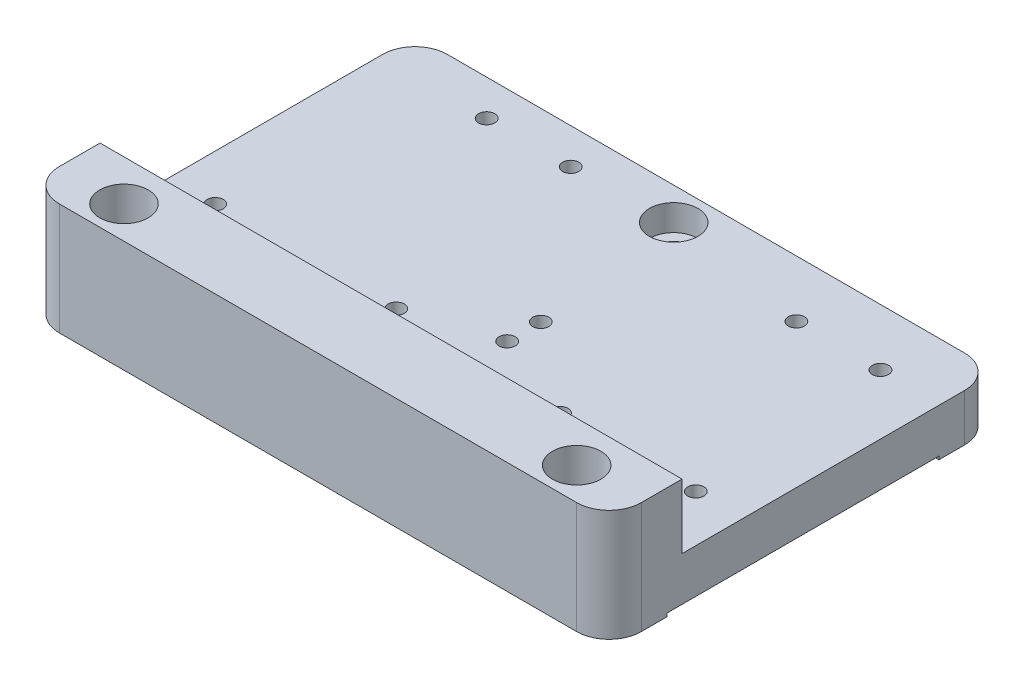
SolidWorks part; units mm, degrees
ref_plane "Front Plane" through (0, 0, 0) normal (0, 0, 1) x (1, 0, 0)
ref_plane "Top Plane" through (0, 0, 0) normal (0, 1, 0) x (1, 0, 0)
ref_plane "Right Plane" through (0, 0, 0) normal (1, 0, 0) x (0, 0, -1)
sketch "Sketch1" plane through (0, 0, 0) normal (0, 1, 0) x (1, 0, 0)
  line L1 (-73.3594, 57.0703) -> (16.6406, 57.0703)
  line L2 (-73.3594, 57.0703) -> (-73.3594, -2.9297)
  line L3 (-73.3594, -2.9297) -> (16.6406, -2.9297)
  line L4 (16.6406, 57.0703) -> (16.6406, -2.9297)
  dimension "D1" = 90
  dimension "D2" = 60
extrude "Boss-Extrude1" add sketch "Sketch1" along normal blind 7.3
sketch "Sketch2" plane through (0, 7.3, 0) normal (0, 1, 0) x (1, 0, 0)
  line L0 (-73.3594, -2.9297) -> (16.6406, -2.9297)
  line L1 (16.6406, -2.9297) -> (16.6406, 8.3703)
  line L2 (16.6406, -2.9297) -> (16.6406, 57.0703) construction
  line L6 (-73.3594, 57.0703) -> (-73.3594, -2.9297) construction
  line L7 (-73.3594, 8.3703) -> (-73.3594, -2.9297)
  line L8 (-73.3594, 8.3703) -> (16.6406, 8.3703)
  dimension "D1" = 11.3
extrude "Boss-Extrude2" add sketch "Sketch2" along normal blind 9.98
hole_wizard "M3 Tapped Hole1" positions "Sketch3" profile "Sketch4" tap size "M3" standard "GB"
sketch "Sketch3" plane through (0, 7.3, 0) normal (0, 1, 0) x (1, 0, 0)
  line L1 (16.6406, 8.3703) -> (16.6406, 57.0703) construction
  line L2 (16.6406, 57.0703) -> (-73.3594, 57.0703) construction
  line L3 (-73.3594, 57.0703) -> (-73.3594, 8.3703) construction
  point P0 (-66.2594, 19.0703)
  point P2 (-38.2594, 19.0703)
  point P4 (-56.7594, 51.5503)
  point P6 (-43.7594, 51.5503)
  point P8 (-5.6194, 48.3003)
  point P10 (7.3806, 48.3003)
  point P12 (-11.6194, 17.7503)
  point P14 (9.3806, 17.7503)
  dimension "D3" = 7.26
  dimension "D4" = 21
  dimension "D5" = 8.77
  dimension "D6" = 8.77
  dimension "D7" = 9.26
  dimension "D8" = 13
  dimension "D9" = 7.1
  dimension "D10" = 28
  dimension "D13" = 5.52
  dimension "D14" = 5.52
  dimension "D15" = 16.6
  dimension "D16" = 13
sketch "Sketch4" plane through (-66.2594, 7.3, -19.0703) normal (1, 0, 0) x (0, 0, 1)
  line L0 (0, 0) -> (0, 8.2511)
  line L1 (0, 8.2511) -> (1.25, 7.5)
  line L2 (1.25, 7.5) -> (1.25, 0)
  line L5 (1.25, 0) -> (0, 0)
  line L10 (0, 8.2511) -> (-1.25, 7.5) construction
  line L11 (0, -6.35) -> (0, 107.95) construction
  dimension "螺纹孔钻头直径" = 2.5
  dimension "螺纹孔钻头深度" = 7.5
  dimension "导头角度" = 118
cosmetic thread "Hole Thread 1" parameters "D1"=6, "D2"=3
cosmetic thread "Hole Thread 2" parameters "D1"=6, "D2"=3
cosmetic thread "Hole Thread 3" parameters "D1"=6, "D2"=3
cosmetic thread "Hole Thread 4" parameters "D1"=6, "D2"=3
cosmetic thread "Hole Thread 5" parameters "D1"=6, "D2"=3
cosmetic thread "Hole Thread 6" parameters "D1"=6, "D2"=3
cosmetic thread "Hole Thread 7" parameters "D1"=6, "D2"=3
cosmetic thread "Hole Thread 8" parameters "D1"=6, "D2"=3
fillet "Fillet1" radius 5 4 edges at (-73.3594, 3.65, -57.0703) (16.6406, 3.65, -57.0703) (16.6406, 8.64, 2.9297) (-73.3594, 8.64, 2.9297)
sketch "Sketch5" plane through (0, 17.28, 0) normal (0, 1, 0) x (1, 0, 0)
  line L0 (-28.3594, -942.9297) -> (-28.3594, 49057.0703) construction
  line L1 (11.6406, 57.0703) -> (-68.3594, 57.0703) construction
  line L2 (-68.3594, -2.9297) -> (11.6406, -2.9297) construction
  line L3 (-73.3594, 8.3703) -> (-73.3594, 2.0703) construction
  circle A0 centre (-28.3594, 52.0703) radius 3.75
  circle A1 centre (-63.3594, 2.0703) radius 3.75
  circle A2 centre (6.6406, 2.0703) radius 3.75
  point P5 (-28.3594, 57.0703)
  dimension "D1" = 5
  dimension "D3" = 7.5
  dimension "D4" = 7.5
  dimension "D2" = 5
  dimension "D5" = 10
extrude "Cut-Extrude1" cut sketch "Sketch5" against normal blind 14
sketch "Sketch6" plane through (0, 3.28, 0) normal (0, 1, 0) x (1, 0, 0)
  circle A0 centre (-28.3594, 52.0703) radius 2.1
  circle A1 centre (-63.3594, 2.0703) radius 2.1
  circle A2 centre (6.6406, 2.0703) radius 2.1
  dimension "D1" = 4.2
  dimension "D2" = 4.2
  dimension "D3" = 4.2
extrude "Cut-Extrude2" cut sketch "Sketch6" against normal through all
sketch "Sketch7" plane through (16.6406, 0, 0) normal (1, 0, 0) x (0, 0, -1)
  line L0 (2.0703, 0) -> (52.0703, 0) construction
  line L1 (6.0703, 0) -> (48.0703, 0)
  line L2 (6.0703, 0) -> (6.0703, 0.5)
  line L3 (6.0703, 0.5) -> (48.0703, 0.5)
  line L4 (48.0703, 0) -> (48.0703, 0.5)
  line L5 (-2.9297, 0) -> (-2.9297, 17.28) construction
  line L6 (57.0703, 7.3) -> (57.0703, 0) construction
  dimension "D1" = 9
  dimension "D2" = 9
  dimension "D3" = 0.5
extrude "Cut-Extrude3" cut sketch "Sketch7" against normal through all
hole_wizard "M3 Tapped Hole3" positions "Sketch10" profile "Sketch11" tap size "M3" standard "GB"
sketch "Sketch10" plane through (0, 7.3, 0) normal (0, 1, 0) x (1, 0, 0)
  point P0 (-24.5694, 11.7703)
  point P3 (-24.5694, 16.9703)
  point P6 (-25.3094, 23.2703)
  point P9 (-25.3094, 28.4703)
sketch "Sketch11" plane through (-24.5694, 7.3, -11.7703) normal (1, 0, 0) x (0, 0, 1)
  line L0 (0, 0) -> (0, 9.2511)
  line L1 (0, 9.2511) -> (1.25, 8.5)
  line L2 (1.25, 8.5) -> (1.25, 0)
  line L5 (1.25, 0) -> (0, 0)
  line L10 (0, 9.2511) -> (-1.25, 8.5) construction
  line L11 (0, -6.35) -> (0, 107.95) construction
  dimension "螺纹孔钻头直径" = 2.5
  dimension "螺纹孔钻头深度" = 8.5
  dimension "导头角度" = 118
cosmetic thread "Hole Thread 13" parameters "D1"=6, "D2"=3
cosmetic thread "Hole Thread 14" parameters "D1"=6, "D2"=3
cosmetic thread "Hole Thread 15" parameters "D1"=6, "D2"=3
cosmetic thread "Hole Thread 16" parameters "D1"=6, "D2"=3
